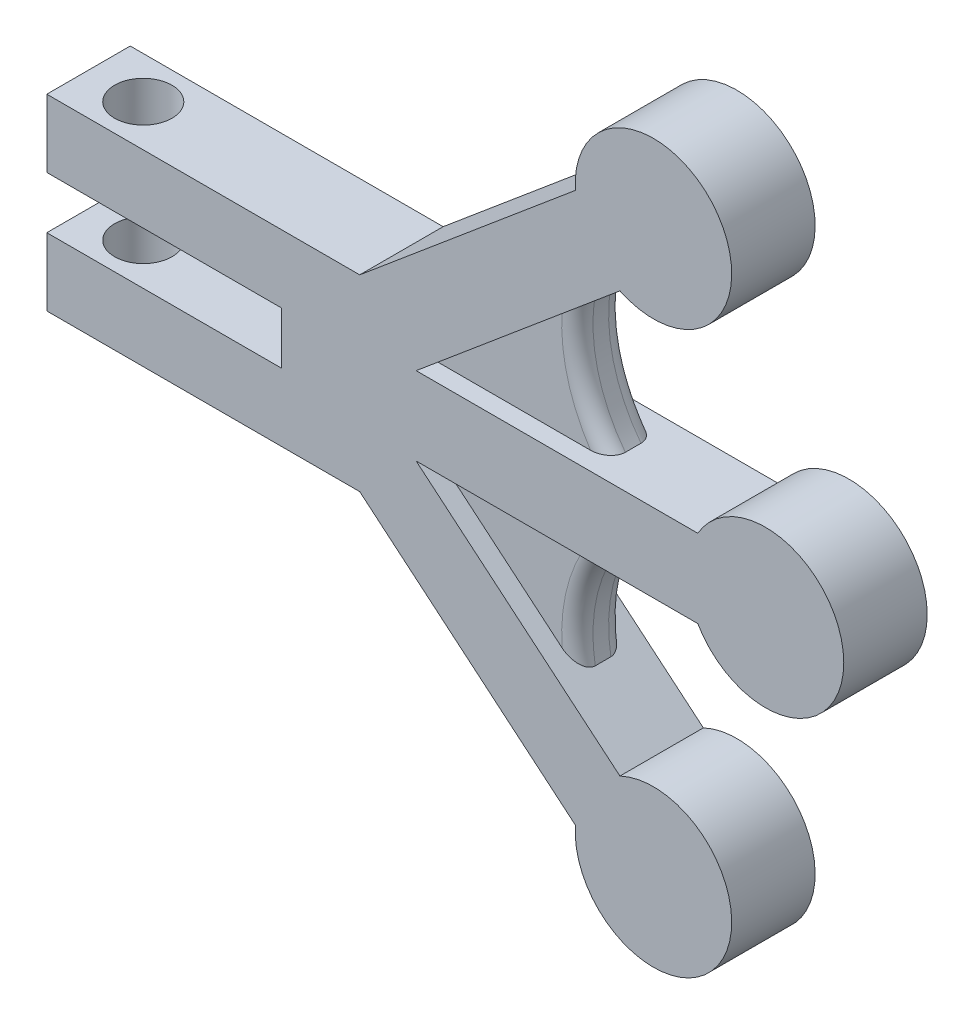
SolidWorks part; units mm, degrees
ref_plane "Alzado" through (0, 0, 0) normal (0, 0, 1) x (1, 0, 0)
ref_plane "Planta" through (0, 0, 0) normal (0, 1, 0) x (1, 0, 0)
ref_plane "Vista lateral" through (0, 0, 0) normal (1, 0, 0) x (0, 0, -1)
sketch "Sketch1" plane through (0, 0, 0) normal (0, 0, 1) x (1, 0, 0)
  line L0 (-20, 0) -> (20, 0) construction
  line L1 (-6, 0) -> (-6, 6)
  line L2 (-6, 6) -> (14, 6)
  line L3 (14, 6) -> (27.7888, 17.5702)
  line L4 (30.6302, 13.4274) -> (17.6075, 2.5)
  line L5 (17.6075, -2.5) -> (35.6075, -2.5)
  line L6 (17.6075, 2.5) -> (35.6075, 2.5)
  line L7 (30.6302, -13.4274) -> (17.6075, -2.5)
  line L8 (14, -6) -> (27.7888, -17.5702)
  line L9 (-6, -6) -> (14, -6)
  line L10 (-6, 0) -> (-6, -6)
  arc A0 (27.7888, 17.5702) -> (30.6302, 13.4274) centre (32.7748, 17.9441) cw
  arc A1 (27.7888, -17.5702) -> (30.6302, -13.4274) centre (32.7748, -17.9441) ccw
  arc A2 (35.6075, 2.5) -> (35.6075, -2.5) centre (39.9376, 0) cw
  dimension "D9" = 5
  dimension "D10" = 5
  dimension "D1" = 40
  dimension "D2" = 5
  dimension "D3" = 18
  dimension "D4" = 18
  dimension "D5" = 6
  dimension "D6" = 17
  dimension "D7" = 140
  dimension "D8" = 20
  dimension "D11" = 6
  dimension "D12" = 5
extrude "Saliente-Extruir1" add sketch "Sketch1" along normal mid plane 8
sketch "Croquis2" plane through (0, 0, 0) normal (0, 0, 1) x (1, 0, 0)
  line L0 (26.8848, 10.2846) -> (14.6281, 0)
  line L1 (17.6075, 2.5) -> (30.6302, 13.4274) construction
  line L2 (14.6281, 0) -> (26.8848, -10.2846)
  line L3 (30.6302, -13.4274) -> (17.6075, -2.5) construction
  arc A0 (26.8848, 10.2846) -> (31.6281, 0) centre (36.7409, 8.5941) ccw
  arc A1 (26.8848, -10.2846) -> (31.6281, 0) centre (36.7409, -8.5941) cw
  dimension "D4" = 10
  dimension "D5" = 10
  dimension "D1" = 16
  dimension "D2" = 14.6281
  dimension "D3" = 17
extrude "Saliente-Extruir2" add sketch "Croquis2" along normal mid plane 3
sketch "Croquis3" plane through (0, 0, 4) normal (0, 0, 1) x (1, 0, 0)
  line L0 (-6, 6) -> (-6, -6) construction
  line L1 (-6, 2) -> (9, 2)
  line L2 (-6, 2) -> (-6, -2)
  line L3 (-6, -2) -> (9, -2)
  line L4 (9, 2) -> (9, -2)
  dimension "D1" = 4
  dimension "D2" = 2
  dimension "D3" = 15
extrude "Cortar-Extruir1" cut sketch "Croquis3" against normal through all
sketch "Croquis4" plane through (0, 6, 0) normal (0, 1, 0) x (1, 0, 0)
  circle A0 centre (-2.5, 0) radius 1.65
  dimension "D1" = 3.3
  dimension "D2" = 2.5
extrude "Cortar-Extruir2" cut sketch "Croquis4" against normal through all
fillet "Fillet2" radius 1 4 edges at (27.034, -6.1906, 1.5) (27.034, -6.1906, -1.5) (27.034, 6.1906, 1.5) (27.034, 6.1906, -1.5)
scale "Scale1" scale about origin uniform scaling yes scale factor 0.3
sketch "Sketch2" plane through (0, 0, 1.2) normal (0, 0, 1) x (1, 0, 0)
  circle A0 centre (0, 0) radius 15.0459
extrude "Cut-Extrude3" cut sketch "Sketch2" against normal blind 0.4
sketch "Sketch3" plane through (0, 0, -1.2) normal (0, 0, -1) x (-1, 0, 0)
  circle A0 centre (0, 0) radius 13.9887
extrude "Cut-Extrude4" cut sketch "Sketch3" against normal blind 0.4
sketch "Sketch4" plane through (0, 0, 0.8) normal (0, 0, 1) x (1, 0, 0)
  line L0 (2.7, 0.6) -> (2.7, -0.6) construction
  line L1 (-1.8, -0.6) -> (2.7, -0.6)
  line L2 (-1.8, -0.6) -> (-1.8, -0.5)
  line L3 (-1.8, -0.5) -> (2.7, -0.5)
  line L4 (2.7, -0.6) -> (2.7, -0.5)
  line L6 (-1.8, 0.6) -> (2.7, 0.6)
  line L7 (-1.8, 0.6) -> (-1.8, 0.5)
  line L8 (-1.8, 0.5) -> (2.7, 0.5)
  line L9 (2.7, 0.6) -> (2.7, 0.5)
  dimension "D1" = 0.5
  dimension "D2" = 0.5
extrude "Boss-Extrude1" add sketch "Sketch4" against normal up to surface (1.6 mm away) up to face at (5.062, 0, -0.8)
sketch "Sketch5" plane through (0, -1.8, 0) normal (0, -1, 0) x (1, 0, 0)
  circle A0 centre (-0.75, 0) radius 0.55
  dimension "D1" = 1.1
extrude "Cut-Extrude5" cut sketch "Sketch5" against normal blind 4.4
